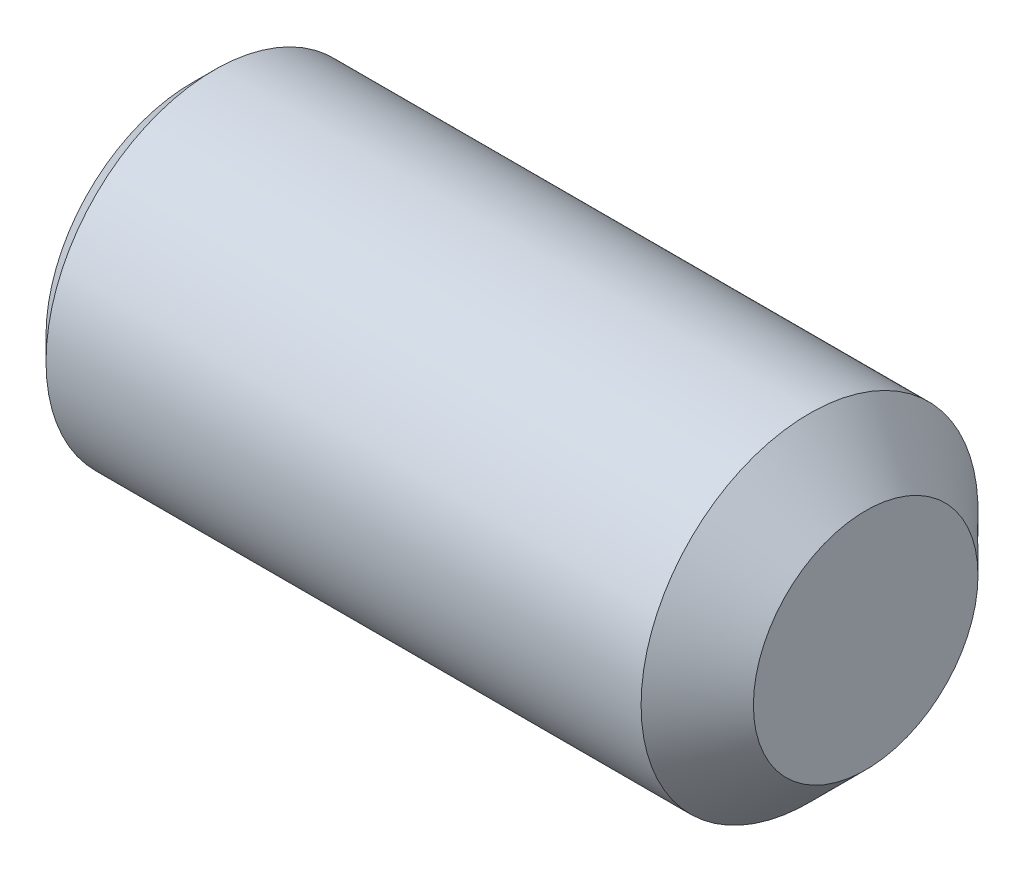
SolidWorks part; units mm, degrees
revolve "Base-Revolve" add sketch "Sketch1" angle 360 about L6
sketch "Sketch1" plane through (0, 0, 0) normal (0, 0, 1) x (1, 0, 0)
  line L0 (0, 0) -> (12, 0)
  line L1 (12, 0) -> (12, 2)
  line L2 (12, 2) -> (11, 3)
  line L3 (11, 3) -> (0.402, 3)
  line L4 (0.402, 3) -> (0, 2.598)
  line L5 (0, 2.598) -> (0, 0)
  line L6 (-0.2778, 0) -> (5.1995, 0) construction
cosmetic thread "Cosmetic Thread1" parameters "df"=5.196
extrude "Cut-Extrude1" cut sketch "Sketch2" against normal blind 2
sketch "Sketch2" plane through (0, 0, 0) normal (-1, 0, 0) x (0, 0, 1)
  line L1 (-0.86, -1.4896) -> (0.86, -1.4896)
  line L2 (0.86, -1.4896) -> (1.72, 0)
  line L3 (1.72, 0) -> (0.86, 1.4896)
  line L4 (0.86, 1.4896) -> (-0.86, 1.4896)
  line L5 (-0.86, 1.4896) -> (-1.72, 0)
  line L6 (-1.72, 0) -> (-0.86, -1.4896)
  circle A0 centre (0, 0) radius 1.4896 construction
material "  "
ref_plane "Front Plane" through (0, 0, 0) normal (0, 0, 1) x (1, 0, 0)
ref_plane "Top Plane" through (0, 0, 0) normal (0, 1, 0) x (1, 0, 0)
ref_plane "Right Plane" through (0, 0, 0) normal (1, 0, 0) x (0, 0, -1)
sketch "Dimension sketch" plane through (0, 0, 0) normal (0, 0, 1) x (1, 0, 0)
  line L0 (0, 0) -> (12, 0)
  point P3 (2, 0)
  point P4 (11, 0)
  point P5 (8, 0)
  point P6 (5.196, 0)
  point P7 (6, 0)
  point P8 (8.56, 0)
sketch "Sketch4" plane through (0, 0, 0) normal (0, 0, 1) x (1, 0, 0)
  line L0 (-0.2778, 0) -> (1.1933, 0) construction
  line L2 (-0.2778, 0) -> (5.1995, 0) construction
  line L3 (2, 1.4896) -> (2.86, 0)
  line L4 (2.86, 0) -> (2, 0)
  line L5 (2, 0) -> (2, 1.4896)
  line L6 (2, 1.4896) -> (0, 1.4896) construction
revolve "Cut-Revolve2" cut sketch "Sketch4" angle 360 about L0
sketch "Sketch5" plane through (0, 0, 0) normal (0, 0, 1) x (1, 0, 0)
  line L0 (0.402, 3) -> (1.402, 3)
  line L1 (11, 3) -> (0.402, 3) construction
  line L2 (1.402, 3) -> (0.8966, 2.134)
  line L3 (0.8966, 2.134) -> (0.402, 3)
  line L5 (5.1995, 0) -> (3.6008, 0) construction
  line L6 (-0.2778, 0) -> (5.1995, 0) construction
  line L7 (0.402, 3) -> (0, 2.598) construction
revolve "Cut-Revolve3" [suppressed] cut sketch "Sketch5" angle 360 about L5
pattern_linear "LPattern1" [suppressed] count 12
equation "\"l@Sketch1\"=\"l@Dimension sketch\""
equation "\"d@Sketch1\"=\"d@Dimension sketch\""
equation "\"df@Sketch1\" = \"df@Dimension sketch\""
equation "\"dp@Sketch1\" = \"dp@Dimension sketch\""
equation "\"e@Sketch2\" = \"e@Dimension sketch\""
equation "\"t@Cut-Extrude1\" = \"t@Dimension sketch\""
equation "\"P@Sketch5\" = \"P@Dimension sketch\""
equation "\"D1@Sketch5\" = \"P@Dimension sketch\"*0.866"
equation "\"P@LPattern1\" = \"P@Dimension sketch\""
equation "\"D1@LPattern1\" = \"l@Dimension sketch\"/\"P@Dimension sketch\""
equation "\"df@Cosmetic Thread1\"=\"df@Dimension sketch\""
equation "\"D2@Sketch4\" = \"t@Dimension sketch\""
